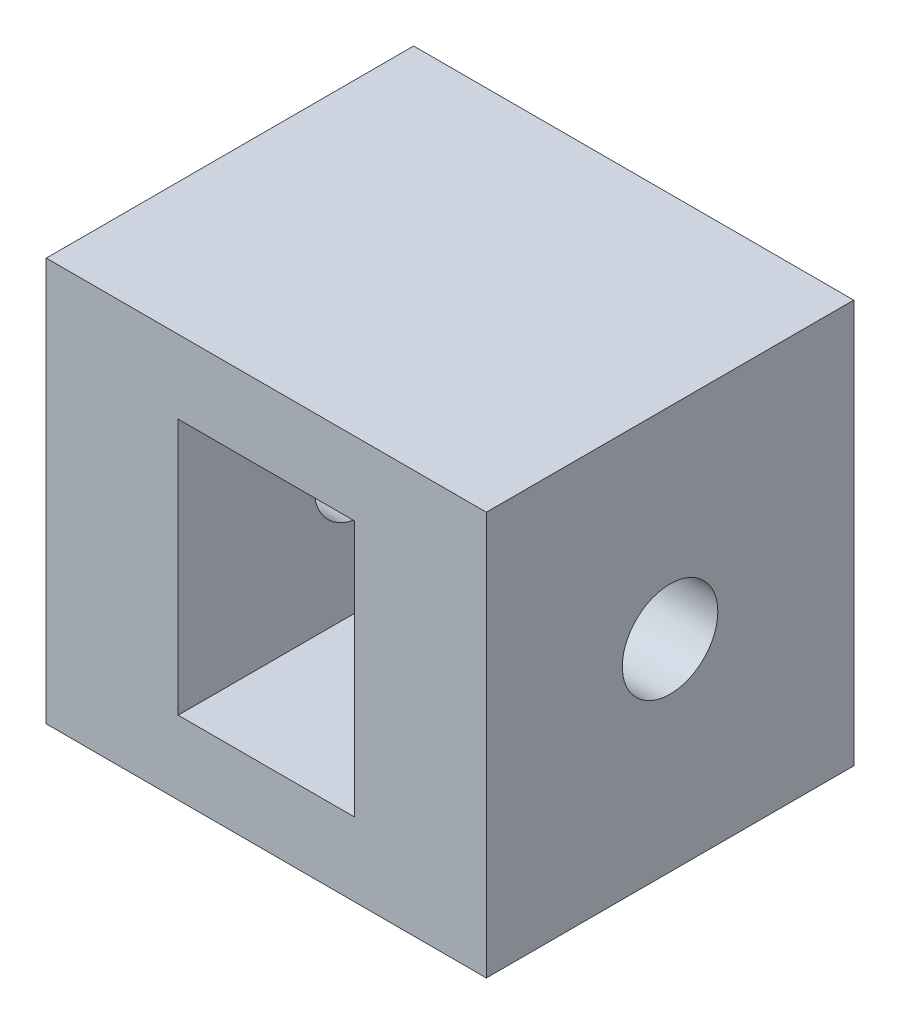
from build123d import *

# Parameters (mm, degrees)
BOSS_EXTRUDE1_DEPTH = 10
SKETCH4_R           = 1.3
CUT_EXTRUDE2_DEPTH  = 19.004466113


with BuildPart() as part:
    # Sketch1 → Boss-Extrude1 (new body)
    with BuildSketch(Plane.XY):
        Polygon((-2, 8.98), (6.39, 8.98), (9.98, 8.98), (9.98, -2), (6.39, -2), (-2, -2), align=None)
        Polygon((1.59, 0), (4.8, 0), (6.39, 0), (6.39, 6.98), (4.8, 6.98), (1.59, 6.98), (1.59, 3.49), align=None, mode=Mode.SUBTRACT)
    extrude(amount=BOSS_EXTRUDE1_DEPTH)

    # Sketch4 → Cut-Extrude2 (cut, through all)
    with BuildSketch(Plane(origin=(9.98, 0, 0), x_dir=(0, 0, -1), z_dir=(1, 0, 0))):
        with Locations((-5, 3.49)):
            Circle(SKETCH4_R)
    extrude(amount=-CUT_EXTRUDE2_DEPTH, mode=Mode.SUBTRACT)


solid = part.part
